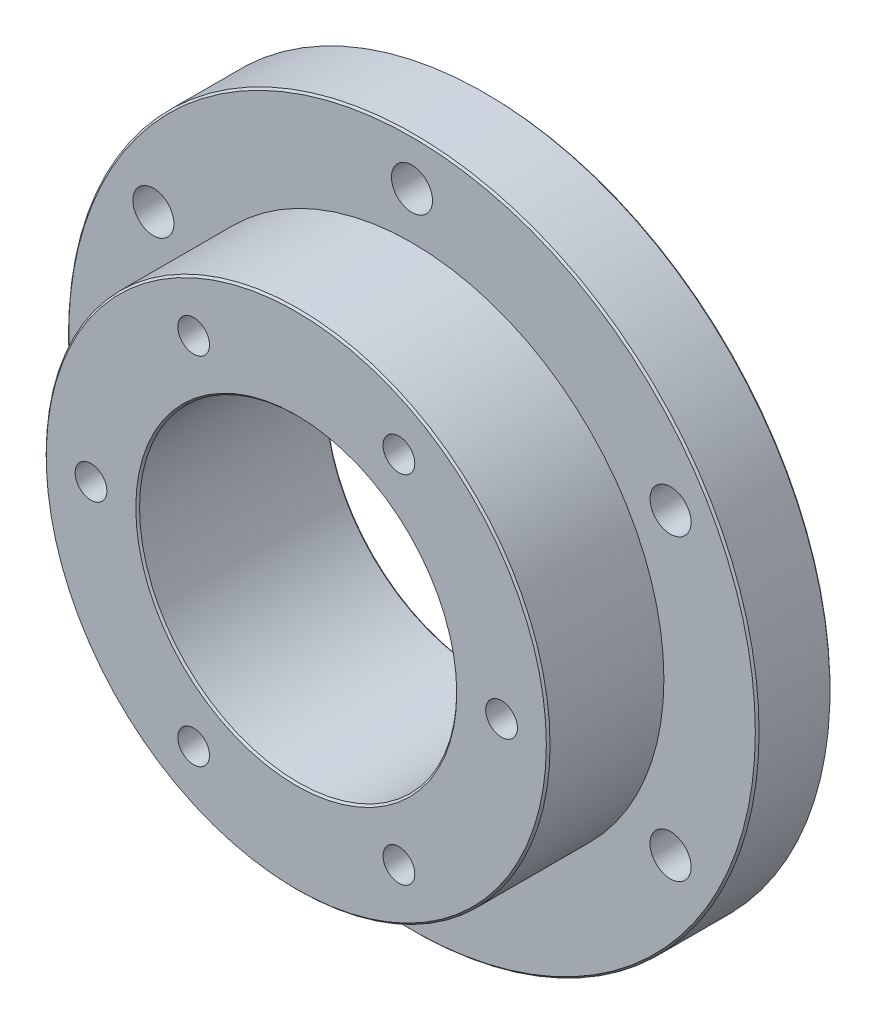
from build123d import *

# Parameters (mm, degrees)
HOLE_WIZARD_1_D           = 11
HOLE_WIZARD_1_CBORE_D     = 18
HOLE_WIZARD_1_CBORE_DEPTH = 11
PATTERN_CIRCULAR_1_COUNT  = 6
PATTERN_CIRCULAR_2_COUNT  = 6
CHAMFER_1_SIZE            = 0.5


with BuildPart() as part:
    # 草图1 → 旋转1 (revolve)
    with BuildSketch(Plane(origin=(0, 0, 0), x_dir=(1, 0, 0), z_dir=(0, 1, 0))):
        Polygon((-42.5, 20), (-42.5, -31), (-67.5, -31), (-67.5, 0), (-92.5, 0), (-92.5, 20), align=None)
    revolve(axis=Axis((0, 0, 0), (0, 0, 1)))

    # 打孔尺寸(%根据)内六角圆柱头螺钉的类型1 (through all)
    with Locations(Plane(origin=(0, 0, -20), x_dir=(1, 0, 0), z_dir=(0, 0, -1))):
        with Locations((0, 80)):
            hole_wizard_1 = CounterBoreHole(HOLE_WIZARD_1_D / 2, HOLE_WIZARD_1_CBORE_D / 2, HOLE_WIZARD_1_CBORE_DEPTH)

    # 阵列(圆周)1: 打孔尺寸(%根据)内六角圆柱头螺钉的类型1 ×6 about axis
    pattern_circular_1_axis = Axis((0, 0, 0), (0, 0, 1))
    for i in range(1, PATTERN_CIRCULAR_1_COUNT):
        add(hole_wizard_1.rotate(pattern_circular_1_axis, i * 360 / PATTERN_CIRCULAR_1_COUNT), mode=Mode.SUBTRACT)

    # 草图7 → M10 螺纹孔1 (revolve, cut)
    with BuildSketch(Plane(origin=(-55, 0, 31), x_dir=(0, -1, 0), z_dir=(1, 0, 0))):
        Polygon((0, 0), (0, 27.053657631), (4.25, 24.5), (4.25, 0), align=None)
    hole_wizard_m10_1 = revolve(axis=Axis((-55, 0, 37.35), (0, 0, -1)), mode=Mode.SUBTRACT)

    # 阵列(圆周)2: M10 螺纹孔1 ×6 about axis
    pattern_circular_2_axis = Axis((0, 0, 0), (0, 0, 1))
    for i in range(1, PATTERN_CIRCULAR_2_COUNT):
        add(hole_wizard_m10_1.rotate(pattern_circular_2_axis, i * 360 / PATTERN_CIRCULAR_2_COUNT), mode=Mode.SUBTRACT)

    # 倒角1
    chamfer_1_edges = [part.edges().sort_by_distance(p)[0] for p in [
        (42.5, 0, 31),
        (42.5, 0, -20),
        (92.5, 0, -20),
        (92.5, 0, 0),
        (67.5, 0, 31),
    ]]
    chamfer(chamfer_1_edges, length=CHAMFER_1_SIZE)


solid = part.part
